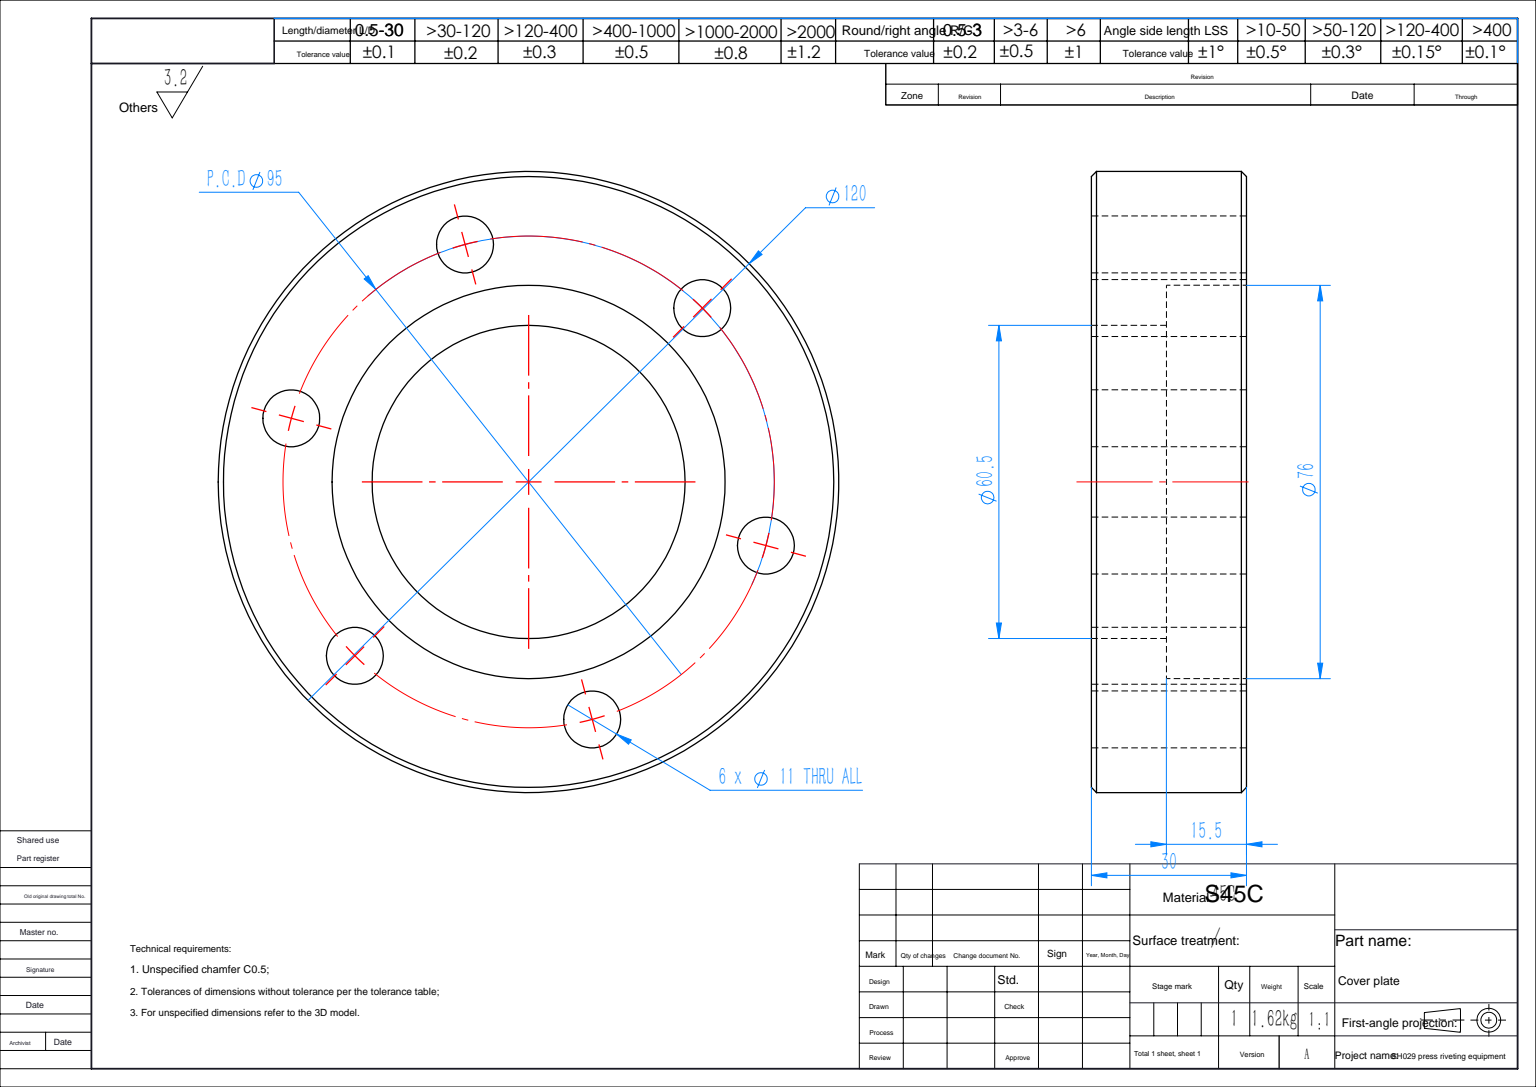
SolidWorks part; units mm, degrees
material "S45C"
ref_plane "前视" through (0, 0, 0) normal (0, 0, 1) x (1, 0, 0)
ref_plane "上视" through (0, 0, 0) normal (0, 1, 0) x (1, 0, 0)
ref_plane "右视" through (0, 0, 0) normal (1, 0, 0) x (0, 0, -1)
sketch "草图1" plane through (0, 0, 0) normal (0, 1, 0) x (1, 0, 0)
  line L0 (0, 222.7151) -> (0, -222.7151) construction
  line L1 (-222.7151, 0) -> (222.7151, 0) construction
  line L2 (-15, 60) -> (15, 60)
  line L3 (15, 60) -> (15, 38)
  line L4 (15, 38) -> (-0.5, 38)
  line L5 (-0.5, 38) -> (-0.5, 30.25)
  line L6 (-0.5, 30.25) -> (-15, 30.25)
  line L7 (-15, 30.25) -> (-15, 60)
  dimension "D1" = 30
  dimension "D2" = 15.5
  dimension "D3" = 120
  dimension "D4" = 76
  dimension "D5" = 60.5
revolve "旋转1" add sketch "草图1" angle 360 about L1
chamfer "倒角1" distance 1 angle 45 2 edges at (15, 0, 60) (-15, 0, 60)
hole_wizard "M10 间隙孔1" positions "草图2" profile "草图3" hole size "M10" standard "GB" end condition through all
sketch "草图2" plane through (-15, 0, 0) normal (-1, 0, 0) x (0, 0, 1)
  line L1 (0, 0) -> (0, -47.5) construction
  line L4 (0, 0) -> (33.5876, -33.5876) construction
  line L5 (0, 30.25) -> (0, 60) construction
  line L8 (0, 45.125) -> (-4.1791, 45.125) construction
  circle A2 centre (0, 0) radius 47.5 construction
  circle A3 centre (0, 0) radius 30.25 construction
  circle A4 centre (0, 0) radius 60 construction
  point P11 (33.5876, -33.5876)
  dimension "D1" = 95
  dimension "D2" = 45
sketch "草图3" plane through (-15, -33.5876, 33.5876) normal (0, 1, 0) x (0, 0, 1)
  line L0 (0, 0) -> (0, 30)
  line L1 (0, 30) -> (5.5, 30)
  line L2 (5.5, 30) -> (5.5, 0)
  line L5 (5.5, 0) -> (0, 0)
  line L11 (0, -6.35) -> (0, 107.95) construction
  dimension "通孔孔直径" = 11
  dimension "通孔孔深度" = 30
pattern_circular "阵列(圆周)1" count 6 over 360 about axis through (0, 0, 0) along (1, 0, 0) of "M10 间隙孔1"
